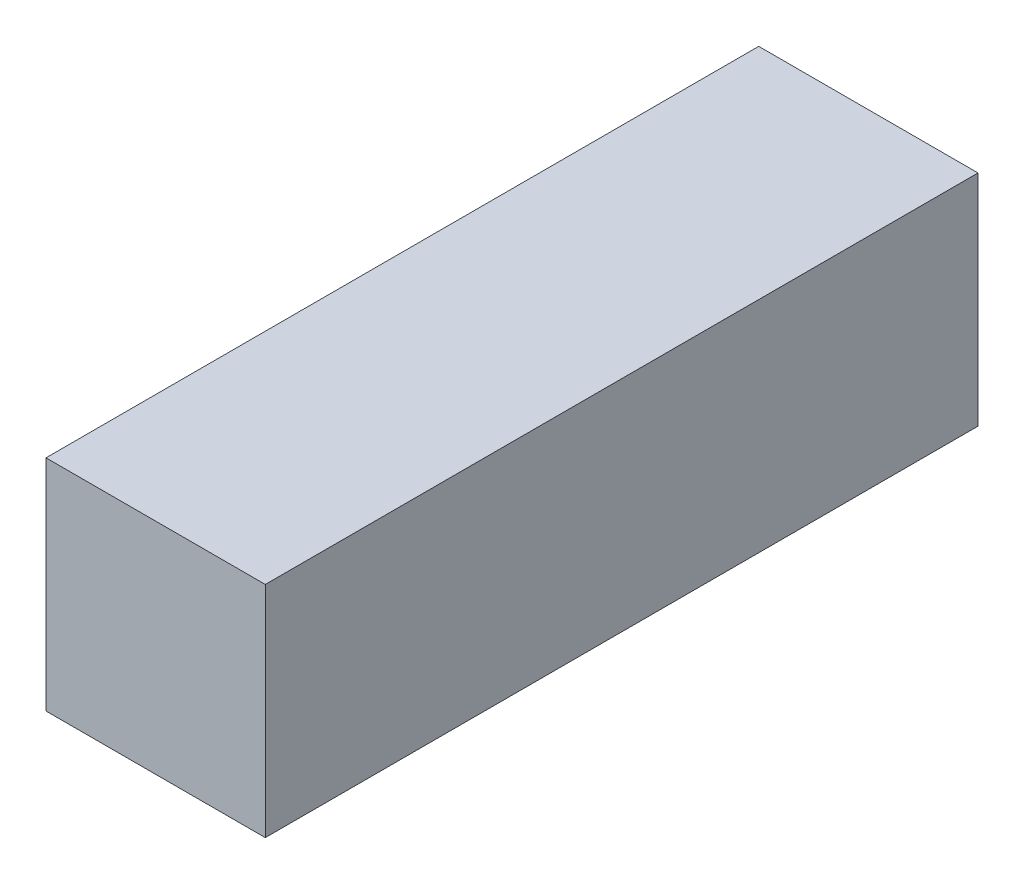
SolidWorks part; units mm, degrees
ref_plane "Front Plane" through (0, 0, 0) normal (0, 0, 1) x (1, 0, 0)
ref_plane "Top Plane" through (0, 0, 0) normal (0, 1, 0) x (1, 0, 0)
ref_plane "Right Plane" through (0, 0, 0) normal (1, 0, 0) x (0, 0, -1)
sketch "Sketch1" plane through (0, 0, 0) normal (0, 1, 0) x (1, 0, 0)
  line L0 (-10, 32.5) -> (10, -32.5) construction
  line L1 (-10, 32.5) -> (10, 32.5)
  line L2 (-10, 32.5) -> (-10, -32.5)
  line L3 (-10, -32.5) -> (10, -32.5)
  line L4 (10, 32.5) -> (10, -32.5)
  dimension "D1" = 20
  dimension "D2" = 65
extrude "Boss-Extrude1" add sketch "Sketch1" along normal blind 20
